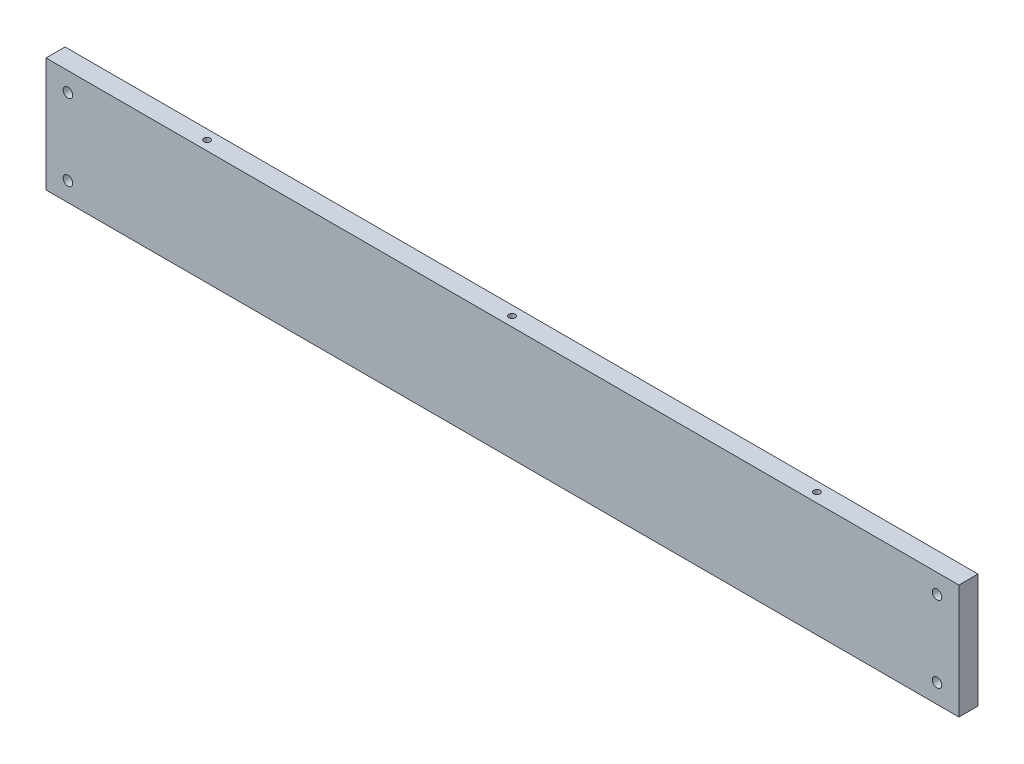
from build123d import *

# Parameters (mm, degrees)
SKETCH_1_W             = 479
SKETCH_1_H             = 10
EXTRUDE_1_DEPTH        = 60
HOLE_WIZARD_M5_1_D     = 4.2
HOLE_WIZARD_M5_1_DEPTH = 12.4
HOLE_WIZARD_M5_1_TIP   = 1.2618073
HOLE_WIZARD_M6_1_D     = 5
HOLE_WIZARD_M4_1_D     = 3.3
HOLE_WIZARD_M4_1_DEPTH = 10.1
HOLE_WIZARD_M4_1_TIP   = 0.991420021


with BuildPart() as part:
    # 草图1 → 凸台-拉伸1 (new body)
    with BuildSketch(Plane(origin=(0, 0, 0), x_dir=(1, 0, 0), z_dir=(0, 1, 0))):
        Rectangle(SKETCH_1_W, SKETCH_1_H)
    extrude(amount=EXTRUDE_1_DEPTH)

    # M5 螺纹孔1
    with Locations(Plane(origin=(0, 0, 0), x_dir=(-1, 0, 0), z_dir=(0, -1, 0))):
        with Locations((0, 0), (-110, 0), (-220, 0), (220, 0), (110, 0)):
            Hole(HOLE_WIZARD_M5_1_D / 2, depth=HOLE_WIZARD_M5_1_DEPTH)
            with Locations((0, 0, -(HOLE_WIZARD_M5_1_DEPTH + HOLE_WIZARD_M5_1_TIP / 2))):  # 118° drill point
                Cone(0, HOLE_WIZARD_M5_1_D / 2, HOLE_WIZARD_M5_1_TIP, mode=Mode.SUBTRACT)

    # M6 螺纹孔1 (through all)
    with Locations(Plane(origin=(0, 0, -5), x_dir=(-1, 0, 0), z_dir=(0, 0, -1))):
        with Locations((228, 50), (228, 10), (-228, 10), (-228, 50)):
            Hole(HOLE_WIZARD_M6_1_D / 2)

    # M4 螺纹孔1
    with Locations(Plane(origin=(0, 60, 0), x_dir=(1, 0, 0), z_dir=(0, 1, 0))):
        with Locations((0, 0), (-160, 0), (160, 0)):
            Hole(HOLE_WIZARD_M4_1_D / 2, depth=HOLE_WIZARD_M4_1_DEPTH)
            with Locations((0, 0, -(HOLE_WIZARD_M4_1_DEPTH + HOLE_WIZARD_M4_1_TIP / 2))):  # 118° drill point
                Cone(0, HOLE_WIZARD_M4_1_D / 2, HOLE_WIZARD_M4_1_TIP, mode=Mode.SUBTRACT)


solid = part.part
